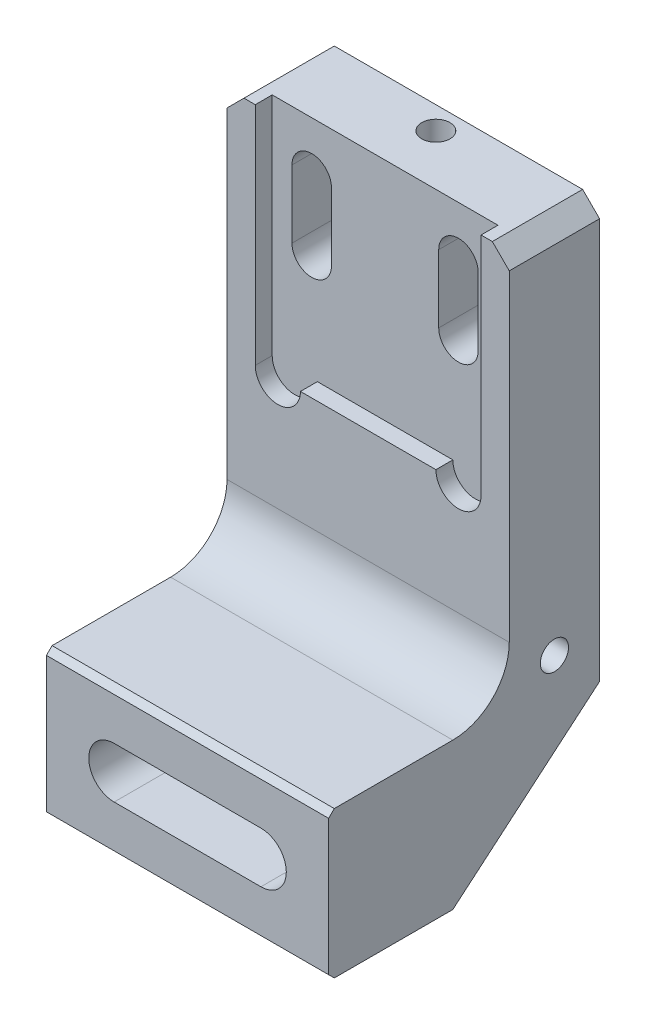
SolidWorks part; units mm, degrees
ref_plane "Front Plane" through (0, 0, 0) normal (0, 0, 1) x (1, 0, 0)
ref_plane "Top Plane" through (0, 0, 0) normal (0, 1, 0) x (1, 0, 0)
ref_plane "Right Plane" through (0, 0, 0) normal (1, 0, 0) x (0, 0, -1)
sketch "Sketch1" plane through (0, 0, 0) normal (0, 0, 1) x (1, 0, 0)
  line L1 (-12.5, -24) -> (12.5, -24)
  line L2 (-12.5, -24) -> (-12.5, 24)
  line L3 (-12.5, 24) -> (12.5, 24)
  line L4 (12.5, -24) -> (12.5, 24)
  line L5 (-12.5, -24) -> (12.5, 24) construction
  line L6 (-12.5, 24) -> (12.5, -24) construction
  point P0 (0, 0)
  dimension "D1" = 25
  dimension "D2" = 48
extrude "Boss-Extrude1" add sketch "Sketch1" along normal mid plane 8
sketch "Sketch5" plane through (0, -24, 0) normal (0, -1, 0) x (1, 0, 0)
  line L0 (12.5, 4) -> (12.5, -4) construction
  line L1 (-12.5, 20) -> (12.5, 20)
  line L2 (-12.5, 20) -> (-12.5, -4)
  line L3 (-12.5, -4) -> (12.5, -4)
  line L4 (12.5, 20) -> (12.5, -4)
  line L5 (-12.5, 20) -> (12.5, -4) construction
  line L6 (-12.5, -4) -> (12.5, 20) construction
  point P0 (0, 8)
  dimension "D1" = 24
extrude "Boss-Extrude3" add sketch "Sketch5" against normal blind 13
sketch "Sketch6" plane through (0, 0, 4) normal (0, 0, 1) x (1, 0, 0)
  line L0 (12.5, 24) -> (-12.5, 24) construction
  line L1 (-10, 4) -> (10, 4)
  line L2 (-10, 4) -> (-10, 44)
  line L3 (-10, 44) -> (10, 44)
  line L4 (10, 4) -> (10, 44)
  line L5 (-10, 4) -> (10, 44) construction
  line L6 (-10, 44) -> (10, 4) construction
  point P0 (0, 24)
  dimension "D1" = 20
  dimension "D2" = 20
extrude "Cut-Extrude1" cut sketch "Sketch6" against normal blind 1.5
hole_wizard "M3 Tapped Hole1" positions "Sketch8" profile "Sketch7" tap size "M3" standard "Gb"
sketch "Sketch8" plane through (0, 24, 0) normal (0, 1, 0) x (1, 0, 0)
  line L0 (0, 0) -> (0, 2) construction
  line L3 (-10, -4) -> (-12.5, -4) construction
  point P0 (0, 2)
  dimension "D1" = 6
sketch "Sketch7" plane through (0, 24, -2) normal (1, 0, 0) x (0, 0, 1)
  line L0 (0, 0) -> (0, 12.2511)
  line L1 (0, 12.2511) -> (1.25, 11.5)
  line L2 (1.25, 11.5) -> (1.25, 0)
  line L5 (1.25, 0) -> (0, 0)
  line L10 (0, 12.2511) -> (-1.25, 11.5) construction
  line L11 (0, -6.35) -> (0, 107.95) construction
  dimension "螺纹孔钻头直径" = 2.5
  dimension "螺纹孔钻头深度" = 11.5
  dimension "导头角度" = 118
cosmetic thread "Cosmetic thread 1" parameters "D1"=10, "D2"=3
chamfer "Chamfer2" distance 1.5 angle 45 2 edges at (12.5, 24, 0) (-12.5, 24, 0)
sketch "Sketch14" plane through (0, 0, -4) normal (0, 0, -1) x (-1, 0, 0)
  line L0 (-6.5, 19.5) -> (-6.5, 13.5) construction
  line L1 (-4.75, 19.5) -> (-4.75, 13.5)
  line L2 (-8.25, 19.5) -> (-8.25, 13.5)
  line L3 (6.5, 19.5) -> (6.5, 13.5) construction
  line L4 (8.25, 19.5) -> (8.25, 13.5)
  line L5 (4.75, 19.5) -> (4.75, 13.5)
  line L6 (0, 24) -> (0, 15.9997) construction
  line L7 (-11, 24) -> (11, 24) construction
  arc A0 (-4.75, 19.5) -> (-8.25, 19.5) centre (-6.5, 19.5) ccw
  arc A1 (-8.25, 13.5) -> (-4.75, 13.5) centre (-6.5, 13.5) ccw
  arc A2 (8.25, 19.5) -> (4.75, 19.5) centre (6.5, 19.5) ccw
  arc A3 (4.75, 13.5) -> (8.25, 13.5) centre (6.5, 13.5) ccw
  point P2 (-6.5, 16.5)
  point P7 (6.5, 16.5)
  dimension "D1" = 3.5
  dimension "D2" = 13
  dimension "D3" = 4.5
  dimension "D4" = 6
extrude "Cut-Extrude3" cut sketch "Sketch14" against normal through all
hole_wizard "M3 Tapped Hole2" positions "Sketch16" profile "Sketch15" tap size "M3" standard "Gb"
sketch "Sketch16" plane through (-12.5, 0, 0) normal (-1, 0, 0) x (0, 0, 1)
  line L0 (0, 22.5) -> (0, -47.404) construction
  line L1 (4, 22.5) -> (-4, 22.5) construction
  line L3 (20, -24) -> (-4, -24) construction
  point P0 (0, -9)
  dimension "D1" = 15
sketch "Sketch15" plane through (-12.5, -9, 0) normal (0, 1, 0) x (0, 0, 1)
  line L0 (0, 0) -> (0, 12.2511)
  line L1 (0, 12.2511) -> (1.25, 11.5)
  line L2 (1.25, 11.5) -> (1.25, 0)
  line L5 (1.25, 0) -> (0, 0)
  line L10 (0, 12.2511) -> (-1.25, 11.5) construction
  line L11 (0, -6.35) -> (0, 107.95) construction
  dimension "螺纹孔钻头直径" = 2.5
  dimension "螺纹孔钻头深度" = 11.5
  dimension "导头角度" = 118
cosmetic thread "Cosmetic thread 2" parameters "D1"=10, "D2"=3
sketch "Sketch18" plane through (0, 0, 4) normal (0, 0, 1) x (1, 0, 0)
  line L0 (-10, 4) -> (10, 4) construction
  line L1 (-10, 4) -> (10, 4) construction
  line L2 (10, 4) -> (10, 24) construction
  line L3 (-10, 24) -> (-10, 4) construction
  circle A0 centre (-8, 4) radius 2
  circle A1 centre (8, 4) radius 2
  dimension "D1" = 4
extrude "Cut-Extrude5" cut sketch "Sketch18" against normal up to surface (1.5 mm away) up to face at (-6.5, 16.5, 2.5)
sketch "Sketch20" plane through (0, 0, -4) normal (0, 0, -1) x (-1, 0, 0)
  line L0 (-6.5, -17.5) -> (6.5, -17.5) construction
  line L1 (-6.5, -15.25) -> (6.5, -15.25)
  line L2 (-6.5, -19.75) -> (6.5, -19.75)
  line L3 (0, -24) -> (0, -17.5) construction
  line L5 (12.5, -24) -> (-12.5, -24) construction
  arc A0 (-6.5, -15.25) -> (-6.5, -19.75) centre (-6.5, -17.5) ccw
  arc A1 (6.5, -19.75) -> (6.5, -15.25) centre (6.5, -17.5) ccw
  point P2 (0, -17.5)
  dimension "D1" = 4.5
  dimension "D2" = 13
  dimension "D3" = 6.5
extrude "Cut-Extrude6" cut sketch "Sketch20" against normal through all
sketch "Sketch21" plane through (12.5, 0, 0) normal (1, 0, 0) x (0, 0, -1)
  line L0 (-9, -24) -> (4, -13)
  line L1 (-20, -24) -> (4, -24) construction
  line L2 (4, -24) -> (4, 22.5) construction
  line L3 (4, -13) -> (4, -24)
  line L4 (4, -24) -> (-9, -24)
  dimension "D1" = 13
  dimension "D2" = 11
extrude "Cut-Extrude7" cut sketch "Sketch21" against normal through all
sketch "Sketch22" plane through (0, 0, -4) normal (0, 0, -1) x (-1, 0, 0)
  line L0 (-6.5, -17.5) -> (6.5, -17.5) construction
  line L1 (-6.5, -13.5) -> (6.5, -13.5)
  line L2 (-6.5, -21.5) -> (6.5, -21.5)
  arc A0 (-6.5, -13.5) -> (-6.5, -21.5) centre (-6.5, -17.5) ccw
  arc A1 (6.5, -21.5) -> (6.5, -13.5) centre (6.5, -17.5) ccw
  point P4 (0, -17.5)
  dimension "D1" = 8
extrude "Cut-Extrude8" cut sketch "Sketch22" against normal offset from surface (15 mm away) 9 up to face at (0, -17.5, 20)
fillet "Fillet2" radius 5 1 edges at (0, -11, 4)
mirror "Mirror1" about plane through (0, 0, 0) normal (1, 0, 0) of "M3 Tapped Hole2"
chamfer "Chamfer4" distance 0.5 angle 45 2 edges at (0, -24, 20) (0, -11, 20)
